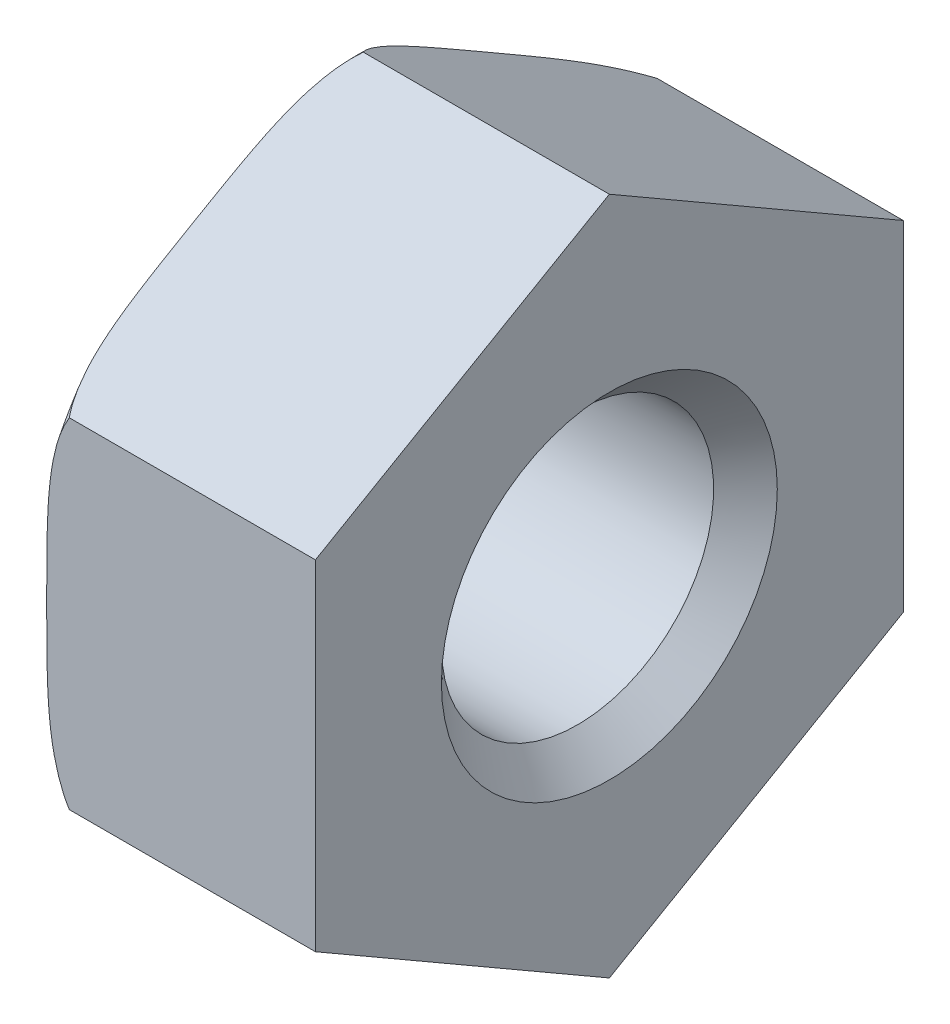
from build123d import *

# Parameters (mm, degrees)
CUT_EXTRUDE1_DEPTH      = 1.6
CUT_EXTRUDE1_DEPTH_BACK = 1.6
SKETCH3_W               = 14
SKETCH3_H               = 14


with BuildPart() as part:
    # Sketch1 → Revolve1 (revolve)
    with BuildSketch(Plane.XY, mode=Mode.PRIVATE) as revolve1_sk:
        with BuildLine():
            Line((-1.6, 0), (-1.6, 3.48))
            ThreePointArc((-1.6, 3.48), (-1.389116882, 3.989116882), (-0.88, 4.2))
            Line((-0.88, 4.2), (1.6, 4.2))
            Line((1.6, 4.2), (1.6, 0))
            Line((1.6, 0), (-1.6, 0))
        make_face()
    revolve(revolve1_sk.sketch.rotate(Axis((1.6, 0, 0), (-1, 0, 0)), 270), axis=Axis((1.6, 0, 0), (-1, 0, 0)))

    # Sketch2 → Cut-Revolve1 (revolve, cut)
    with BuildSketch(Plane.XY, mode=Mode.PRIVATE) as cut_revolve1_sk:
        Polygon((-1.6, 0), (-1.6, 2), (-1.221, 1.621), (1.221, 1.621), (1.6, 2), (1.6, 0), align=None)
    revolve(cut_revolve1_sk.sketch.rotate(Axis((1.6, 0, 0), (-1, 0, 0)), 270), axis=Axis((1.6, 0, 0), (-1, 0, 0)), mode=Mode.SUBTRACT)

    # Sketch3 → Cut-Extrude1 (cut, two sides: drawn at the far end of the back side and taken through both)
    with BuildSketch(Plane(origin=(0, 0, 0), x_dir=(0, 0, -1), z_dir=(1, 0, 0)).offset(-CUT_EXTRUDE1_DEPTH_BACK)):
        Rectangle(SKETCH3_W, SKETCH3_H)
        Polygon((-3.5, 2.020725942), (-3.5, -2.020725942), (0, -4.041451884), (3.5, -2.020725942), (3.5, 2.020725942), (0, 4.041451884), align=None, mode=Mode.SUBTRACT)
    extrude(amount=CUT_EXTRUDE1_DEPTH + CUT_EXTRUDE1_DEPTH_BACK, mode=Mode.SUBTRACT)


solid = part.part
